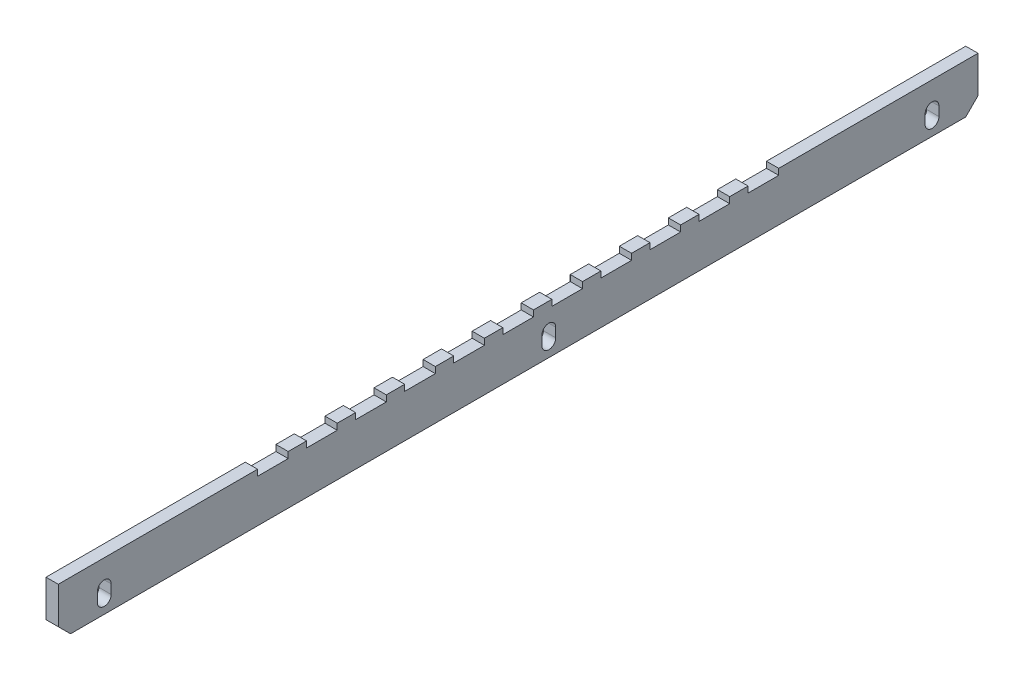
from build123d import *

# Parameters (mm, degrees)
SKETCH_1_W                 = 300
SKETCH_1_H                 = 16
BOSS_EXTRUDE_1_DEPTH       = 4
CHAMFER_1_SIZE             = 4
CUT_EXTRUDE_1_DEPTH        = 151.26643005
SKETCH_3_W                 = 10
SKETCH_3_H                 = 4
CUT_EXTRUDE_2_DEPTH        = 151.26643005
LINEAR_PATTERN_1_COUNT     = 6
LINEAR_PATTERN_1_PITCH     = 16
LINEAR_PATTERN_1_COL_COUNT = 6
LINEAR_PATTERN_1_COL_PITCH = 16
CUT_EXTRUDE_3_DEPTH        = 151.26643005


with BuildPart() as part:
    # Sketch 1 → Boss-Extrude 1 (new body)
    with BuildSketch(Plane(origin=(0, 0, 0), x_dir=(0, 0, -1), z_dir=(1, 0, 0))):
        Rectangle(SKETCH_1_W, SKETCH_1_H)
    extrude(amount=BOSS_EXTRUDE_1_DEPTH)

    # Chamfer 1
    chamfer_1_edges = [part.edges().sort_by_distance(p)[0] for p in [
        (2, -8, -150),
        (2, -8, 150),
    ]]
    chamfer(chamfer_1_edges, length=CHAMFER_1_SIZE)

    # Sketch 2 → Cut-Extrude 1 (cut, through all)
    with BuildSketch(Plane(origin=(4, 0, 0), x_dir=(0, 0, -1), z_dir=(1, 0, 0))):
        with BuildLine():
            Line((-132.75, -0.5), (-132.75, -3.5))
            ThreePointArc((-132.75, -3.5), (-135, -5.75), (-137.25, -3.5))
            Line((-137.25, -3.5), (-137.25, -0.5))
            ThreePointArc((-137.25, -0.5), (-135, 1.75), (-132.75, -0.5))
        make_face()
    cut_extrude_1 = extrude(amount=-CUT_EXTRUDE_1_DEPTH, mode=Mode.SUBTRACT)

    # Mirror 1: Cut-Extrude 1 across plane
    add(cut_extrude_1.mirror(Plane.XY), mode=Mode.SUBTRACT)

    # Sketch 3 → Cut-Extrude 2 (cut, through all)
    with BuildSketch(Plane(origin=(4, 0, 0), x_dir=(0, 0, -1), z_dir=(1, 0, 0))):
        with Locations((0, 8)):
            Rectangle(SKETCH_3_W, SKETCH_3_H)
    cut_extrude_2 = extrude(amount=-CUT_EXTRUDE_2_DEPTH, mode=Mode.SUBTRACT)

    # Linear Pattern 1: Cut-Extrude 2 ×6
    with Locations(*[(0, 0, -i * LINEAR_PATTERN_1_PITCH) for i in range(1, LINEAR_PATTERN_1_COUNT)]):
        add(cut_extrude_2, mode=Mode.SUBTRACT)

    # Linear Pattern 1 col: Cut-Extrude 2 ×6
    with Locations(*[(0, 0, i * LINEAR_PATTERN_1_COL_PITCH) for i in range(1, LINEAR_PATTERN_1_COL_COUNT)]):
        add(cut_extrude_2, mode=Mode.SUBTRACT)

    # Sketch 4 → Cut-Extrude 3 (cut, through all)
    with BuildSketch(Plane(origin=(4, 0, 0), x_dir=(0, 0, -1), z_dir=(1, 0, 0))):
        with BuildLine():
            Line((12.25, -0.5), (12.25, -3.5))
            ThreePointArc((12.25, -3.5), (10, -5.75), (7.75, -3.5))
            Line((7.75, -3.5), (7.75, -0.5))
            ThreePointArc((7.75, -0.5), (10, 1.75), (12.25, -0.5))
        make_face()
    extrude(amount=-CUT_EXTRUDE_3_DEPTH, mode=Mode.SUBTRACT)


solid = part.part
